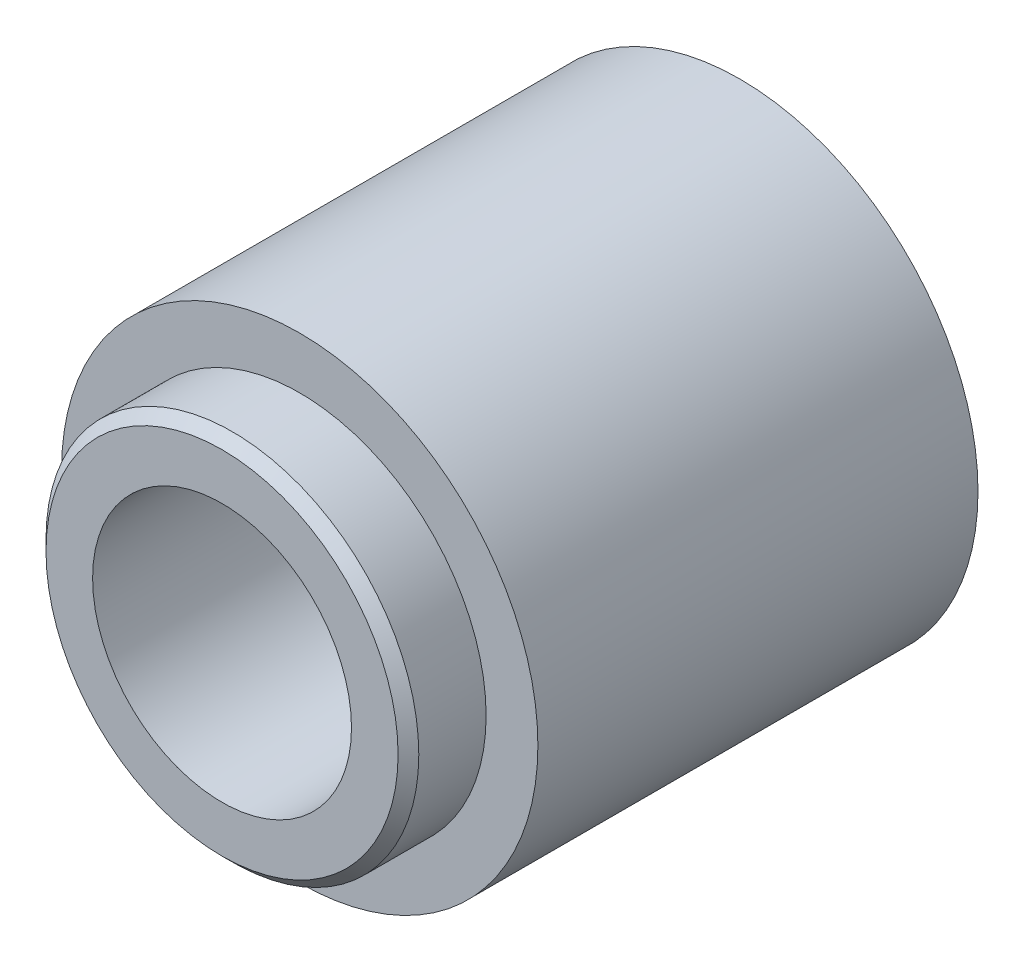
SolidWorks part; units mm, degrees
ref_plane "Front Plane" through (0, 0, 0) normal (0, 0, 1) x (1, 0, 0)
ref_plane "Top Plane" through (0, 0, 0) normal (0, 1, 0) x (1, 0, 0)
ref_plane "Right Plane" through (0, 0, 0) normal (1, 0, 0) x (0, 0, -1)
sketch "Sketch1" plane through (0, 0, 0) normal (0, 0, 1) x (1, 0, 0)
  circle A0 centre (0, 0) radius 23
  dimension "D1" = 46
extrude "Boss-Extrude1" add sketch "Sketch1" along normal blind 50
sketch "Sketch2" plane through (0, 0, 50) normal (0, 0, 1) x (1, 0, 0)
  circle A0 centre (0, 0) radius 23
  circle A1 centre (0, 0) radius 18
  dimension "D1" = 36
extrude "Cut-Extrude1" cut sketch "Sketch2" against normal blind 7.5
sketch "Sketch3" plane through (0, 0, 50) normal (0, 0, 1) x (1, 0, 0)
  circle A0 centre (0, 0) radius 12.5
  dimension "D1" = 25
extrude "Cut-Extrude2" cut sketch "Sketch3" against normal through all
chamfer "Chamfer1" distance 1 angle 45 1 edges at (18, 0, 50)
